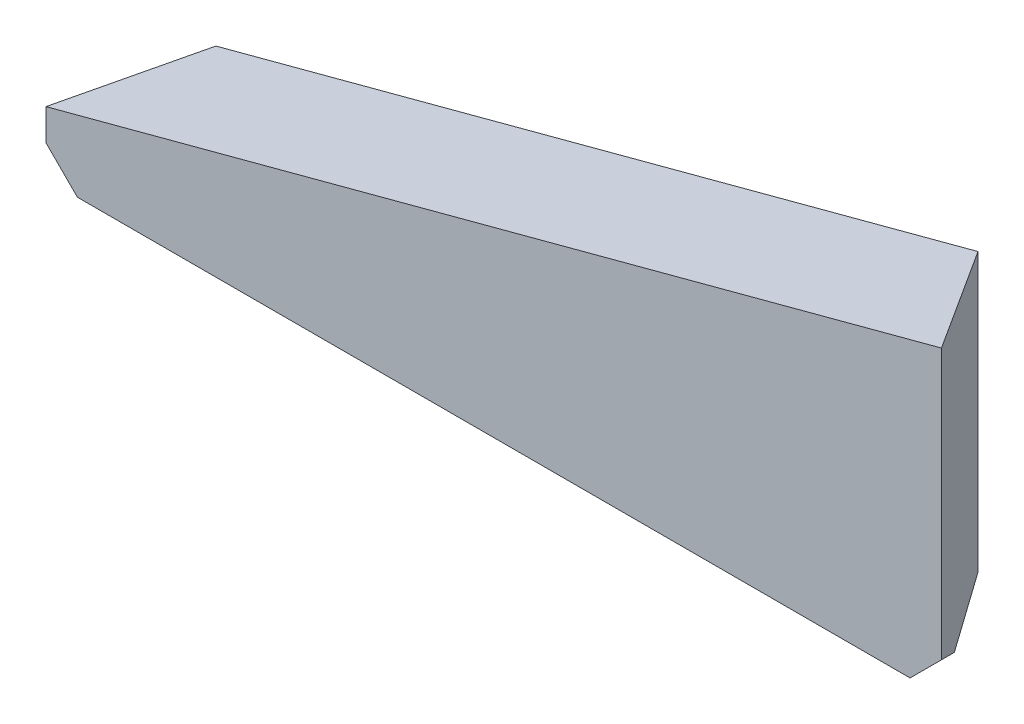
from build123d import *

# Parameters (mm, degrees)
BOSS_EXTRUDE1_DEPTH = 20
CUT_EXTRUDE2_DEPTH  = 50


with BuildPart() as part:
    # Sketch1 → Boss-Extrude1 (new body)
    with BuildSketch(Plane.XY):
        Polygon((5, 0), (137.6, 0), (142.6, 5), (142.6, 48), (0, 10), (0, 5), align=None)
    extrude(amount=BOSS_EXTRUDE1_DEPTH)

    # Sketch2 → Cut-Extrude2 (cut, along a direction that is not the sketch's normal)
    with BuildSketch(Plane(origin=(-2.488112271, 9.33696868, 0), x_dir=(0.9662799118048497, 0.25749394564224604, 0), z_dir=(-0.257493945642246, 0.9662799118048496, 0))):
        Polygon((2.574939456, -20), (9.874939456, 0), (2.574939456, 0), align=None)
        Polygon((150.151224814, -20), (135.474939456, 0), (150.151224814, 0), align=None)
    extrude(amount=-CUT_EXTRUDE2_DEPTH, dir=(0, 1, 0), mode=Mode.SUBTRACT)


solid = part.part
